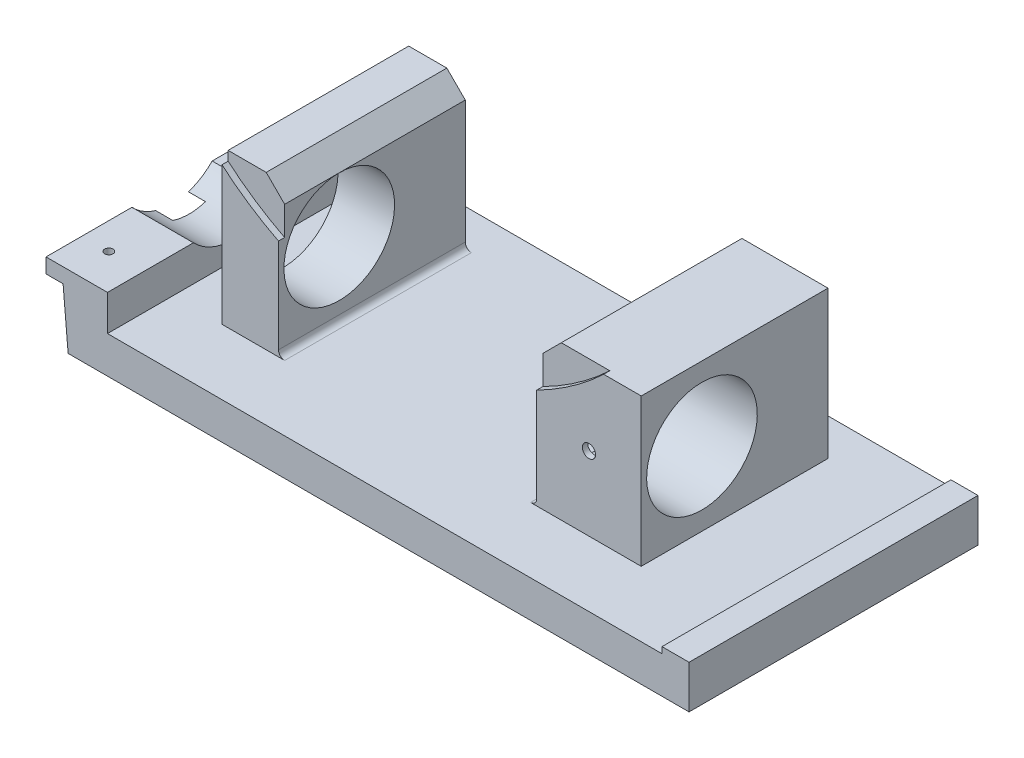
from build123d import *

# Parameters (mm, degrees)
BOSS_EXTRUDE1_DEPTH     = 205
FILLET1_R               = 5
SKETCH2_R               = 45
CUT_EXTRUDE1_DEPTH      = 582.424113707
CUT_EXTRUDE2_DEPTH      = 380.537876952
CUT_EXTRUDE3_DEPTH      = 5
CUT_EXTRUDE3_DEPTH_BACK = 354.691405041
SKETCH5_R               = 232
BOSS_EXTRUDE2_DEPTH     = 30
CUT_EXTRUDE4_DEPTH      = 53.1
M8_TAPPED_HOLE1_D       = 6.8
M8_TAPPED_HOLE1_DEPTH   = 20.207073895
M8_TAPPED_HOLE1_TIP     = 2.042926105


with BuildPart() as part:
    # Sketch1 → Boss-Extrude1 (new body)
    with BuildSketch(Plane.XY):
        with BuildLine():
            Line((-227.111967186, 47), (-223, 0))
            Line((-223, 0), (282, 0))
            Line((282, 0), (282, 35))
            Line((282, 35), (260, 35))
            Line((260, 35), (260, 30))
            Line((260, 30), (190, 30))
            Line((190, 30), (190, 150))
            Line((190, 150), (107.739268607, 150))
            ThreePointArc((107.739268607, 150), (106.373112603, 149.134239248), (105, 148.279554695))
            Line((105, 148.279554695), (105, 30))
            Line((105, 30), (-105, 30))
            Line((-105, 30), (-105, 148.279554695))
            ThreePointArc((-105, 148.279554695), (-106.373112603, 149.134239248), (-107.739268607, 150))
            Line((-107.739268607, 150), (-151, 150))
            Line((-151, 150), (-151, 30))
            Line((-151, 30), (-191, 30))
            Line((-191, 30), (-191, 59))
            Line((-191, 59), (-241, 59))
            Line((-241, 59), (-241, 47))
            Line((-241, 47), (-227.111967186, 47))
        make_face()
    extrude(amount=-BOSS_EXTRUDE1_DEPTH)

    # Fillet1
    fillet1_edges = [part.edges().sort_by_distance(p)[0] for p in [
        (-105, 30, -102.5),
        (105, 30, -102.5),
    ]]
    fillet(fillet1_edges, radius=FILLET1_R)

    # Sketch2 → Cut-Extrude1 (cut, through all)
    with BuildSketch(Plane(origin=(282, 0, 0), x_dir=(0, 0, -1), z_dir=(1, 0, 0))):
        with Locations((102.5, 90)):
            Circle(SKETCH2_R)
    extrude(amount=-CUT_EXTRUDE1_DEPTH, mode=Mode.SUBTRACT)

    # Sketch3 → Cut-Revolve1 (revolve, cut)
    with BuildSketch(Plane(origin=(147.5, 0, 0), x_dir=(0, 0, -1), z_dir=(1, 0, 0)), mode=Mode.PRIVATE) as cut_revolve1_sk:
        Polygon((0, 95.9), (0, 90), (90, 90), (90, 95), align=None)
    revolve(cut_revolve1_sk.sketch.rotate(Axis((147.5, 90, -102.5), (0, 0, 1)), 136.455003644), axis=Axis((147.5, 90, -102.5), (0, 0, 1)), mode=Mode.SUBTRACT)

    # Sketch4 → Cut-Extrude2 (cut, through all)
    with BuildSketch(Plane(origin=(0, 0, -205), x_dir=(-1, 0, 0), z_dir=(0, 0, -1))):
        Polygon((-120, 150), (-105, 135), (-105, 150), align=None)
        Polygon((105, 150), (120, 150), (105, 135), align=None)
    extrude(amount=-CUT_EXTRUDE2_DEPTH, mode=Mode.SUBTRACT)

    # Sketch5 → Cut-Extrude3 (cut, two sides: drawn at the far end of the back side and taken through both)
    with BuildSketch(Plane(origin=(0, 0, -53.1), x_dir=(-1, 0, 0), z_dir=(0, 0, -1)).offset(-CUT_EXTRUDE3_DEPTH_BACK)):
        with Locations((0, 318.5)):
            Circle(SKETCH5_R)
    extrude(amount=CUT_EXTRUDE3_DEPTH + CUT_EXTRUDE3_DEPTH_BACK, mode=Mode.SUBTRACT)

    # Sketch6 → Boss-Extrude2 (add)
    with BuildSketch(Plane(origin=(0, 0, -205), x_dir=(-1, 0, 0), z_dir=(0, 0, -1))):
        Polygon((-282, 0), (223, 0), (227.111967186, 47), (241, 47), (241, 59), (191, 59), (191, 30), (-260, 30), (-260, 35), (-282, 35), align=None)
    extrude(amount=BOSS_EXTRUDE2_DEPTH)

    # Sketch7 → Cut-Extrude4 (cut)
    with BuildSketch(Plane.XY):
        Polygon((-151, 30), (-151, 146.183263941), (-120, 150), (-105, 135), (-105, 35), (-100, 30), align=None)
        Polygon((190, 150), (190, 30), (100, 30), (105, 35), (105, 135), (120, 150), align=None)
    extrude(amount=-CUT_EXTRUDE4_DEPTH, mode=Mode.SUBTRACT)

    # M8 Tapped Hole1
    with Locations(Plane(origin=(0, 59, 0), x_dir=(1, 0, 0), z_dir=(0, 1, 0))):
        with Locations((271, 29.3636836), (271, 219.953225124), (-219.303225542, 219.998090208), (-219.303225542, 29.3636836)):
            Hole(M8_TAPPED_HOLE1_D / 2, depth=M8_TAPPED_HOLE1_DEPTH)
            with Locations((0, 0, -(M8_TAPPED_HOLE1_DEPTH + M8_TAPPED_HOLE1_TIP / 2))):  # 118° drill point
                Cone(0, M8_TAPPED_HOLE1_D / 2, M8_TAPPED_HOLE1_TIP, mode=Mode.SUBTRACT)


solid = part.part
